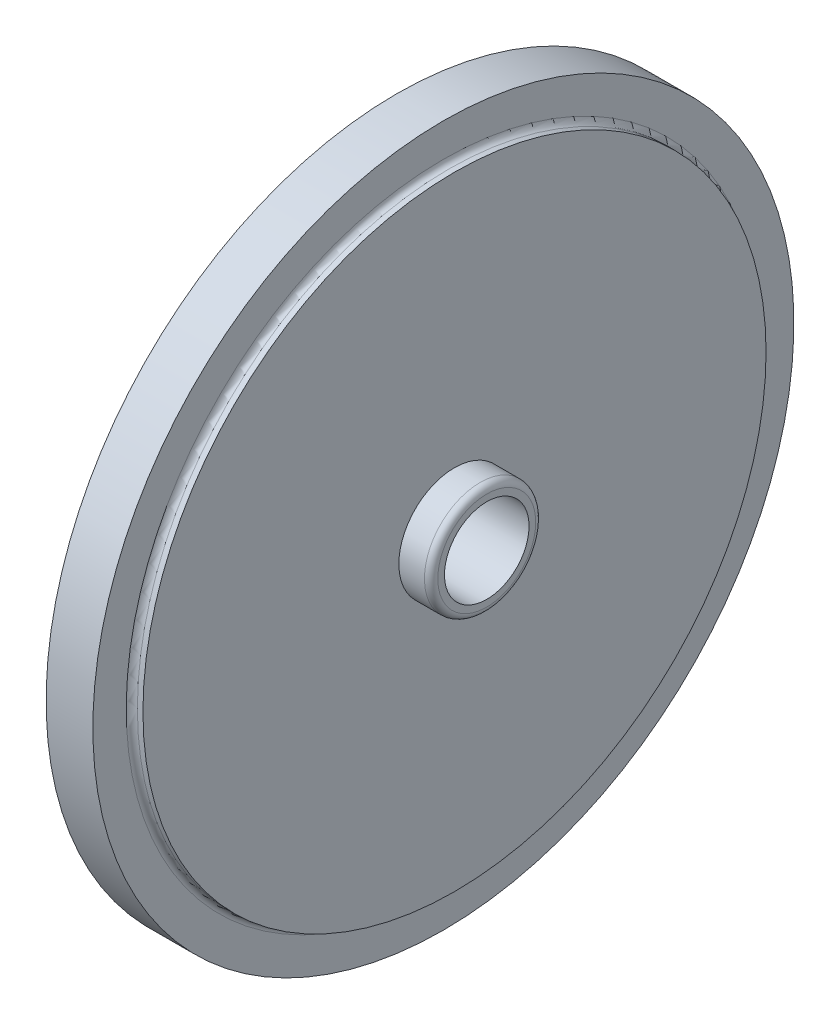
SolidWorks part; units mm, degrees
ref_plane "Front Plane" through (0, 0, 0) normal (0, 0, 1) x (1, 0, 0)
ref_plane "Top Plane" through (0, 0, 0) normal (0, 1, 0) x (1, 0, 0)
ref_plane "Right Plane" through (0, 0, 0) normal (1, 0, 0) x (0, 0, -1)
other "Configuration Table"
sketch "Sketch1" plane through (0, 0, 0) normal (0, 0, 1) x (1, 0, 0)
  line L0 (-55, 0) -> (-417.3463, 0) construction
  line L2 (-130.8, 157.5) -> (-151.8, 157.5)
  line L3 (-150.8, 141.5) -> (-151.8, 141.5)
  line L4 (-125.8, 140) -> (-125.8, 82.5)
  line L5 (-130.8, 157.5) -> (-130.8, 142.5)
  line L6 (-137.8, 107) -> (-137.8, 82.5)
  line L7 (-149.8, 140.5) -> (-149.8, 131.985)
  line L8 (-151.8, 157.5) -> (-151.8, 145.5)
  line L9 (-151.8, 145.5) -> (-151.8, 141.5)
  line L10 (-125.8, 140) -> (-128.3, 140)
  line L11 (-147.3, 22) -> (-147.3, 19)
  line L12 (-111.3, 22) -> (-111.3, 19)
  line L13 (-114.3, 25) -> (-125.8, 25)
  line L14 (-137.8, 25) -> (-144.3, 25)
  line L15 (-137.8, 82.5) -> (-137.8, 25)
  line L16 (-125.8, 82.5) -> (-125.8, 25)
  line L17 (-147.3, 19) -> (-111.3, 19)
  arc A0 (-149.8, 140.5) -> (-150.8, 141.5) centre (-150.8, 140.5) ccw
  arc A1 (-137.8, 107) -> (-149.4251, 131.2045) centre (-168.8104, 107) ccw
  arc A2 (-149.8, 131.985) -> (-149.4251, 131.2045) centre (-148.8, 131.985) ccw
  arc A3 (-130.8, 142.5) -> (-128.3, 140) centre (-128.3, 142.5) ccw
  arc A4 (-144.3, 25) -> (-147.3, 22) centre (-144.3, 22) ccw
  arc A5 (-111.3, 22) -> (-114.3, 25) centre (-114.3, 22) ccw
revolve "Revolve1" add sketch "Sketch1" angle 360 about L0
